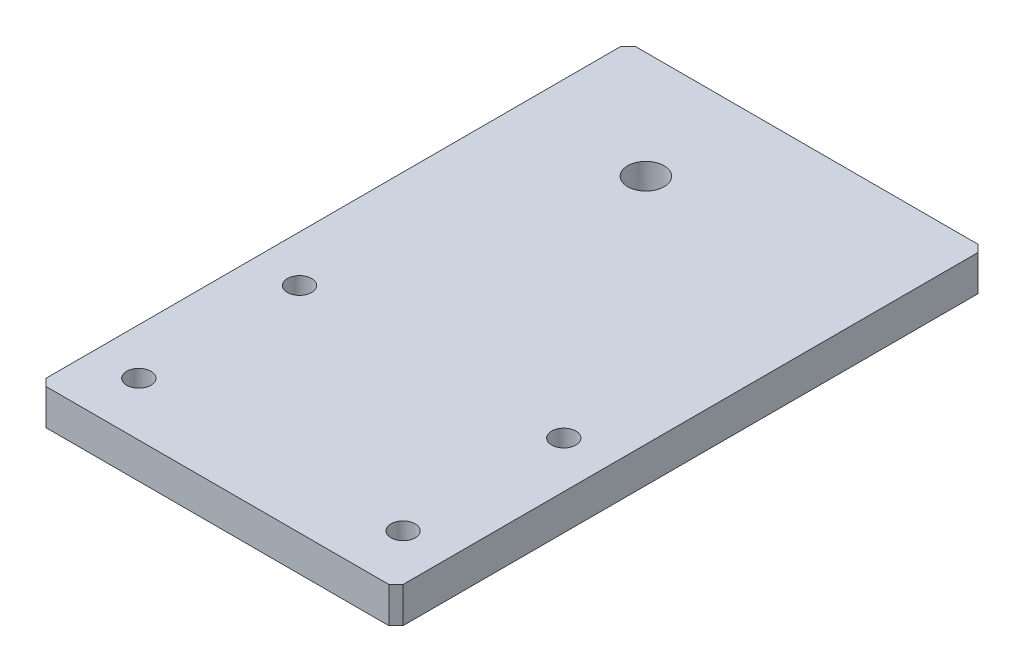
SolidWorks part; units mm, degrees
material "Q235"
ref_plane "前视基准面" through (0, 0, 0) normal (0, 0, 1) x (1, 0, 0)
ref_plane "上视基准面" through (0, 0, 0) normal (0, 1, 0) x (1, 0, 0)
ref_plane "右视基准面" through (0, 0, 0) normal (1, 0, 0) x (0, 0, -1)
sketch "草图1" plane through (0, 0, 0) normal (0, 1, 0) x (1, 0, 0)
  line L1 (0, 0) -> (100, 0)
  line L2 (0, 0) -> (0, 165)
  line L3 (0, 165) -> (100, 165)
  line L4 (100, 0) -> (100, 165)
  dimension "D1" = 100
  dimension "D2" = 165
extrude "凸台-拉伸1" add sketch "草图1" along normal blind 10
chamfer "倒角1" distance 2 angle 45 4 edges at (100, 5, 0) (0, 5, 0) (100, 5, -165) (0, 5, -165)
hole_wizard "M12 螺纹孔1" positions "3D草图1" profile "草图2" tap size "M12" standard "GB"
sketch3d "3D草图1"
  point P0 (35, 10, -135)
  dimension "D1" = 35
  dimension "D2" = 30
sketch "草图2" plane through (35, 10, -135) normal (1, 0, 0) x (0, 0, 1)
  line L0 (0, 0) -> (0, 35.8144)
  line L1 (0, 35.8144) -> (5.1, 32.75)
  line L2 (5.1, 32.75) -> (5.1, 0)
  line L5 (5.1, 0) -> (0, 0)
  line L10 (0, 35.8144) -> (-5.1, 32.75) construction
  line L11 (0, -6.35) -> (0, 107.95) construction
  dimension "螺纹孔钻头直径" = 10.2
  dimension "螺纹孔钻头深度" = 32.75
  dimension "导头角度" = 118
cosmetic thread "孔螺蚊线1" parameters "D1"=10, "D2"=12
hole_wizard "M8 螺纹孔1" positions "3D草图2" profile "草图3" tap size "M8" standard "GB"
sketch3d "3D草图2"
  point P0 (76.5, 10, -41)
  point P2 (76.5, 10, -6)
  point P4 (23.5, 10, -41)
  point P6 (23.5, 10, -6)
  dimension "D1" = 53
  dimension "D2" = 35
  dimension "D3" = 35
  dimension "D4" = 53
  dimension "D5" = 23.5
  dimension "D6" = 23.5
  dimension "D7" = 6
  dimension "D8" = 6
sketch "草图3" plane through (76.5, 10, -41) normal (1, 0, 0) x (0, 0, 1)
  line L0 (0, 0) -> (0, 24.2929)
  line L1 (0, 24.2929) -> (3.4, 22.25)
  line L2 (3.4, 22.25) -> (3.4, 0)
  line L5 (3.4, 0) -> (0, 0)
  line L10 (0, 24.2929) -> (-3.4, 22.25) construction
  line L11 (0, -6.35) -> (0, 107.95) construction
  dimension "螺纹孔钻头直径" = 6.8
  dimension "螺纹孔钻头深度" = 22.25
  dimension "导头角度" = 118
cosmetic thread "孔螺蚊线2" [suppressed] parameters "D1"=10, "D2"=8
cosmetic thread "孔螺蚊线3" [suppressed] parameters "D1"=10, "D2"=8
cosmetic thread "孔螺蚊线4" [suppressed] parameters "D1"=10, "D2"=8
cosmetic thread "孔螺蚊线5" [suppressed] parameters "D1"=10, "D2"=8
hole_wizard "M8 螺纹孔2" positions "草图5" profile "草图4" tap size "M8" standard "GB"
sketch "草图5" plane through (0, 10, 0) normal (0, 1, 0) x (1, 0, 0)
  line L0 (50, 165) -> (50, 0)
  line L1 (98, 165) -> (2, 165) construction
  line L2 (2, 0) -> (98, 0) construction
  point P0 (13, 60)
  point P2 (13, 15)
  point P16 (87, 15)
  point P17 (87, 60)
  dimension "D1" = 45
  dimension "D2" = 37
  dimension "D3" = 15
sketch "草图4" plane through (13, 10, -60) normal (1, 0, 0) x (0, 0, 1)
  line L0 (0, 0) -> (0, 24.2929)
  line L1 (0, 24.2929) -> (3.4, 22.25)
  line L2 (3.4, 22.25) -> (3.4, 0)
  line L5 (3.4, 0) -> (0, 0)
  line L10 (0, 24.2929) -> (-3.4, 22.25) construction
  line L11 (0, -6.35) -> (0, 107.95) construction
  dimension "螺纹孔钻头直径" = 6.8
  dimension "螺纹孔钻头深度" = 22.25
  dimension "导头角度" = 118
cosmetic thread "孔螺蚊线6" parameters "D1"=10, "D2"=8
cosmetic thread "孔螺蚊线7" parameters "D1"=10, "D2"=8
cosmetic thread "孔螺蚊线8" parameters "D1"=10, "D2"=8
cosmetic thread "孔螺蚊线9" parameters "D1"=10, "D2"=8
